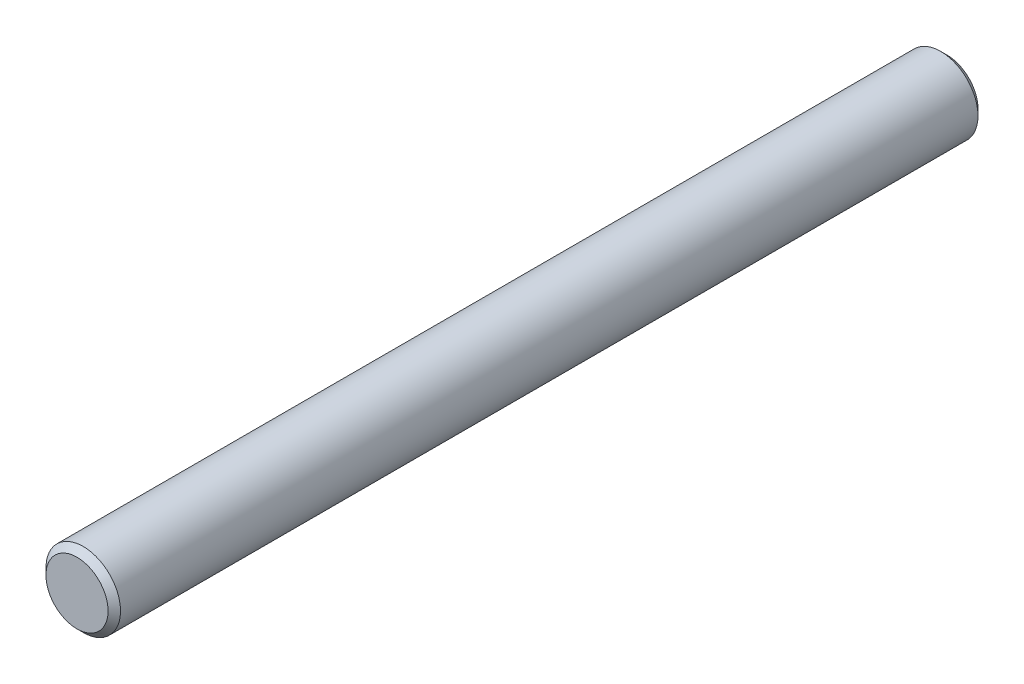
from build123d import *

# Parameters (mm, degrees)
SKETCH1_R           = 3
BOSS_EXTRUDE1_DEPTH = 70
CHAMFER1_SIZE       = 0.5


with BuildPart() as part:
    # Sketch1 → Boss-Extrude1 (new body)
    with BuildSketch(Plane.XY):
        with Locations((81.000178314, -185.451853844)):
            Circle(SKETCH1_R)
    extrude(amount=-BOSS_EXTRUDE1_DEPTH)

    # Chamfer1
    chamfer1_edges = [part.edges().sort_by_distance(p)[0] for p in [
        (78.000178314, -185.451853844, 0),
        (78.000178314, -185.451853844, -70),
    ]]
    chamfer(chamfer1_edges, length=CHAMFER1_SIZE)


solid = part.part
